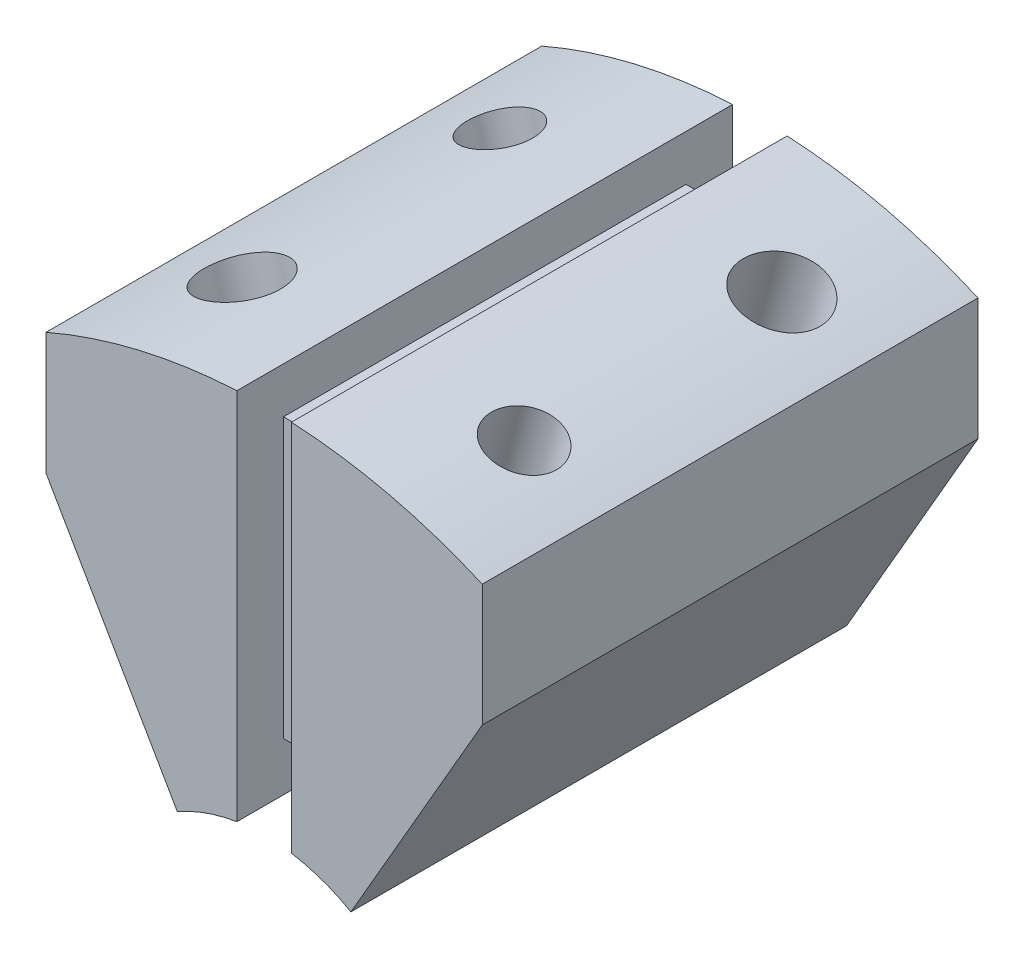
from build123d import *

# Parameters (mm, degrees)
BOSS_EXTRUDE1_DEPTH                       = 25
BOSS_EXTRUDE1_2_DEPTH                     = 25
SKETCH2_W                                 = 5.5
SKETCH2_H                                 = 28.1
BOSS_EXTRUDE2_DEPTH                       = 20.3
F_8_0MM_BLIND_DOWEL_HOLE1_D               = 8
F_8_0MM_BLIND_DOWEL_HOLE1_DEPTH           = 15
F_8_0MM_BLIND_DOWEL_HOLE1_TIP             = 2.403442476
F_8_0MM_BLIND_DOWEL_HOLE1_ON_FACE_2_D     = 8
F_8_0MM_BLIND_DOWEL_HOLE1_ON_FACE_2_DEPTH = 15
F_8_0MM_BLIND_DOWEL_HOLE1_ON_FACE_2_TIP   = 2.403442476
M8_TAPPED_HOLE1_D                         = 6.8
M8_TAPPED_HOLE1_DEPTH                     = 18
M8_TAPPED_HOLE1_TIP                       = 2.042926105
M8_TAPPED_HOLE1_ON_FACE_2_D               = 6.8
M8_TAPPED_HOLE1_ON_FACE_2_DEPTH           = 18
M8_TAPPED_HOLE1_ON_FACE_2_TIP             = 2.042926105


with BuildPart() as part:
    # Sketch1 → Boss-Extrude1 (new, symmetric)
    with BuildSketch(Plane.XY):
        with BuildLine():
            Line((-8.75, 15.155444566), (-22, 38.105117767))
            Line((-22, 38.105117767), (-22, 50.408332645))
            ThreePointArc((-22, 50.408332645), (-12.579933349, 53.541995452), (-2.75, 54.931206977))
            Line((-2.75, 54.931206977), (-2.75, 17.282577933))
            ThreePointArc((-2.75, 17.282577933), (-5.847535728, 16.494130044), (-8.75, 15.155444566))
        make_face()
    extrude(amount=BOSS_EXTRUDE1_DEPTH, both=True)



with BuildPart() as body_2:
    # Sketch1 → Boss-Extrude1 2 (new, symmetric)
    with BuildSketch(Plane.XY):
        with BuildLine():
            Line((8.75, 15.155444566), (22, 38.105117767))
            Line((22, 38.105117767), (22, 50.408332645))
            ThreePointArc((22, 50.408332645), (12.579933349, 53.541995452), (2.75, 54.931206977))
            Line((2.75, 54.931206977), (2.75, 17.282577933))
            ThreePointArc((2.75, 17.282577933), (5.847535728, 16.494130044), (8.75, 15.155444566))
        make_face()
    extrude(amount=BOSS_EXTRUDE1_2_DEPTH, both=True)


with BuildPart() as part_1:
    add(part.part)

    add(body_2.part)  # Boss-Extrude2 merges body 2
    # Sketch2 → Boss-Extrude2 (add, symmetric)
    with BuildSketch(Plane.XY):
        with Locations((0, 36.25)):
            Rectangle(SKETCH2_W, SKETCH2_H)
    extrude(amount=BOSS_EXTRUDE2_DEPTH, both=True)

    # Ø8.0mm Blind Dowel Hole1
    with Locations(Plane(origin=(-14.235047481, 53.125920446, 13), x_dir=(0.965925826289, 0.258819045103, 0), z_dir=(-0.258819045103, 0.965925826289, 0))):
        with Locations((0, 0)):
            Hole(F_8_0MM_BLIND_DOWEL_HOLE1_D / 2, depth=F_8_0MM_BLIND_DOWEL_HOLE1_DEPTH)
            with Locations((0, 0, -(F_8_0MM_BLIND_DOWEL_HOLE1_DEPTH + F_8_0MM_BLIND_DOWEL_HOLE1_TIP / 2))):  # 118° drill point
                Cone(0, F_8_0MM_BLIND_DOWEL_HOLE1_D / 2, F_8_0MM_BLIND_DOWEL_HOLE1_TIP, mode=Mode.SUBTRACT)

    # Ø8.0mm Blind Dowel Hole1 on face 2
    with Locations(Plane(origin=(14.235047481, 53.125920446, -13), x_dir=(0.965925849201, -0.258818959594, 0), z_dir=(0.258818959594, 0.965925849201, 0))):
        with Locations((0, 0)):
            Hole(F_8_0MM_BLIND_DOWEL_HOLE1_ON_FACE_2_D / 2, depth=F_8_0MM_BLIND_DOWEL_HOLE1_ON_FACE_2_DEPTH)
            with Locations((0, 0, -(F_8_0MM_BLIND_DOWEL_HOLE1_ON_FACE_2_DEPTH + F_8_0MM_BLIND_DOWEL_HOLE1_ON_FACE_2_TIP / 2))):  # 118° drill point
                Cone(0, F_8_0MM_BLIND_DOWEL_HOLE1_ON_FACE_2_D / 2, F_8_0MM_BLIND_DOWEL_HOLE1_ON_FACE_2_TIP, mode=Mode.SUBTRACT)

    # M8 Tapped Hole1
    with Locations(Plane(origin=(-14.235047481, 53.125920446, -13), x_dir=(0.965925826289, 0.258819045103, 0), z_dir=(-0.258819045103, 0.965925826289, 0))):
        with Locations((0, 0)):
            Hole(M8_TAPPED_HOLE1_D / 2, depth=M8_TAPPED_HOLE1_DEPTH)
            with Locations((0, 0, -(M8_TAPPED_HOLE1_DEPTH + M8_TAPPED_HOLE1_TIP / 2))):  # 118° drill point
                Cone(0, M8_TAPPED_HOLE1_D / 2, M8_TAPPED_HOLE1_TIP, mode=Mode.SUBTRACT)

    # M8 Tapped Hole1 on face 2
    with Locations(Plane(origin=(14.235047481, 53.125920446, 13), x_dir=(0.965925849201, -0.258818959594, 0), z_dir=(0.258818959594, 0.965925849201, 0))):
        with Locations((0, 0)):
            Hole(M8_TAPPED_HOLE1_ON_FACE_2_D / 2, depth=M8_TAPPED_HOLE1_ON_FACE_2_DEPTH)
            with Locations((0, 0, -(M8_TAPPED_HOLE1_ON_FACE_2_DEPTH + M8_TAPPED_HOLE1_ON_FACE_2_TIP / 2))):  # 118° drill point
                Cone(0, M8_TAPPED_HOLE1_ON_FACE_2_D / 2, M8_TAPPED_HOLE1_ON_FACE_2_TIP, mode=Mode.SUBTRACT)


solid = part_1.part
